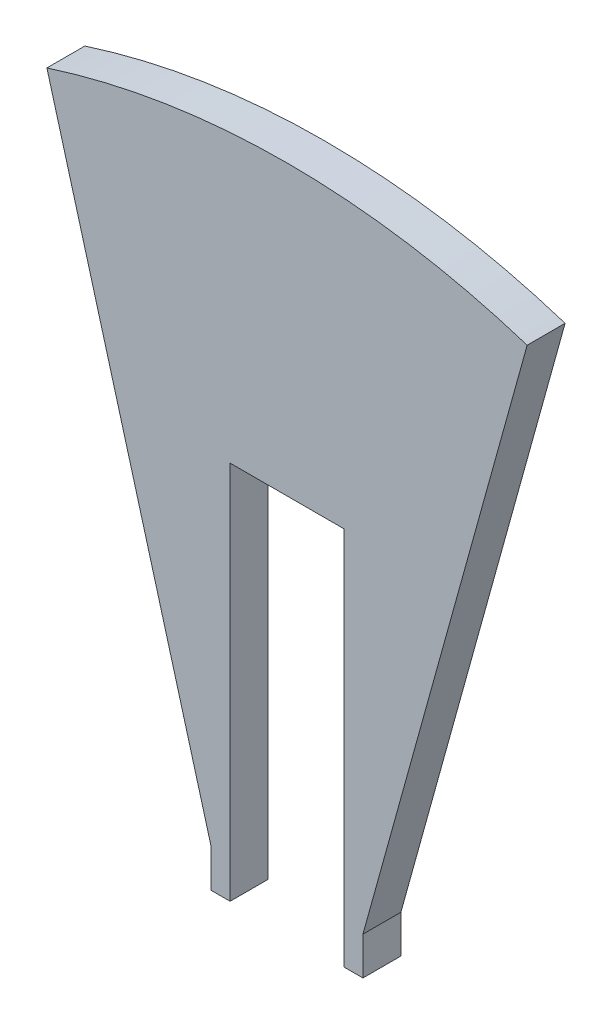
SolidWorks part; units mm, degrees
ref_plane "Front Plane" through (0, 0, 0) normal (0, 0, 1) x (1, 0, 0)
ref_plane "Top Plane" through (0, 0, 0) normal (0, 1, 0) x (1, 0, 0)
ref_plane "Right Plane" through (0, 0, 0) normal (1, 0, 0) x (0, 0, -1)
sketch "Sketch1" plane through (0, 0, 0) normal (0, 0, 1) x (1, 0, 0)
  line L0 (-63.2742, 196.0418) -> (-20, 40)
  line L1 (-20, 40) -> (-20, 30)
  line L2 (-20, 30) -> (20, 30)
  line L3 (20, 30) -> (20, 40)
  line L4 (20, 40) -> (63.2742, 196.0418)
  line L5 (0, 206) -> (0, 0) construction
  arc A0 (63.2742, 196.0418) -> (-63.2742, 196.0418) centre (0, 0) ccw
  dimension "D3" = 30
  dimension "D4" = 412
  dimension "D1" = 40
  dimension "D2" = 10
  dimension "D5" = 31
extrude "Boss-Extrude1" add sketch "Sketch1" along normal mid plane 10
sketch "Sketch2" plane through (0, 0, 5) normal (0, 0, 1) x (1, 0, 0)
  line L0 (-20, 30) -> (20, 30) construction
  line L1 (15, -70) -> (-15, -70)
  line L2 (15, -70) -> (15, 130)
  line L3 (15, 130) -> (-15, 130)
  line L4 (-15, -70) -> (-15, 130)
  line L5 (15, -70) -> (-15, 130) construction
  line L6 (15, 130) -> (-15, -70) construction
  point P0 (0, 30)
  dimension "D1" = 30
  dimension "D2" = 100
extrude "Cut-Extrude1" cut sketch "Sketch2" against normal blind 10
